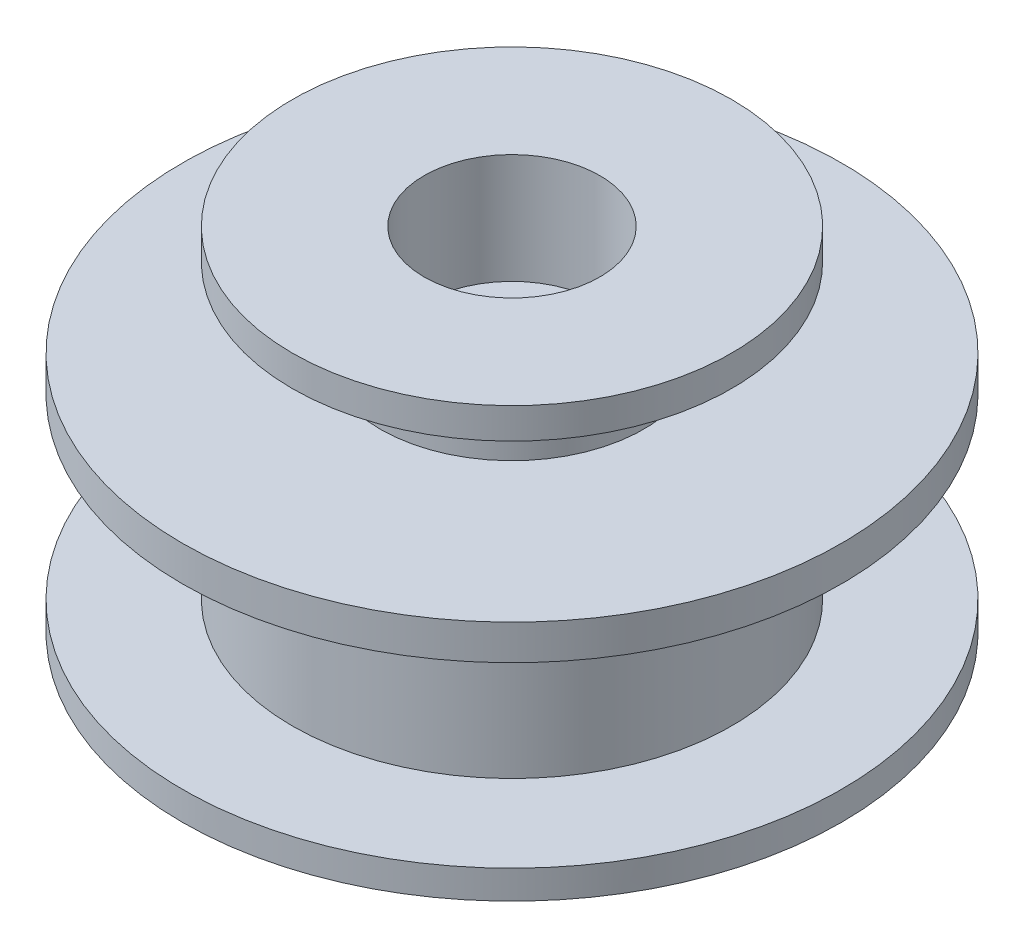
SolidWorks part; units mm, degrees
ref_plane "Front Plane" through (0, 0, 0) normal (0, 0, 1) x (1, 0, 0)
ref_plane "Top Plane" through (0, 0, 0) normal (0, 1, 0) x (1, 0, 0)
ref_plane "Right Plane" through (0, 0, 0) normal (1, 0, 0) x (0, 0, -1)
other "Configuration Table"
sketch "Sketch1" plane through (0, 0, 0) normal (0, 1, 0) x (1, 0, 0)
  circle A0 centre (0, 0) radius 7.5
  dimension "D1" = 15
extrude "Boss-Extrude1" add sketch "Sketch1" along normal blind 4
sketch "Sketch3" plane through (0, 0, 0) normal (0, 0, 1) x (1, 0, 0)
  line L0 (7.5, 0) -> (7.5, 4) construction
  line L1 (7.5, 3.9) -> (4.5, 3.9)
  line L2 (7.5, 3.9) -> (7.5, 0.65)
  line L3 (7.5, 0.65) -> (4.5, 0.65)
  line L4 (4.5, 3.9) -> (4.5, 0.65)
  line L5 (7.5, 4) -> (-7.5, 4) construction
  line L6 (-7.5, 0) -> (7.5, 0) construction
  line L7 (0, 0) -> (0, 7.7691) construction
  dimension "D1" = 0.1
  dimension "D2" = 0.65
  dimension "D3" = 3
revolve "Cut-Revolve1" cut sketch "Sketch3" angle 360 about L7
sketch "Sketch4" plane through (0, 0, 0) normal (0, 1, 0) x (1, 0, 0)
  circle A0 centre (0, 0) radius 5
  dimension "D1" = 10
extrude "Boss-Extrude2" add sketch "Sketch4" along normal blind 8
sketch "Sketch5" plane through (0, 0, 0) normal (0, 0, 1) x (1, 0, 0)
  line L0 (5, 4) -> (5, 8) construction
  line L1 (5, 5.5) -> (3, 5.5)
  line L2 (5, 5.5) -> (5, 7.3)
  line L3 (5, 7.3) -> (3, 7.3)
  line L4 (3, 5.5) -> (3, 7.3)
  line L5 (5, 8) -> (-5, 8) construction
  line L6 (7.5, 4) -> (-7.5, 4) construction
  line L7 (0, 4) -> (0, 7.4809) construction
  dimension "D1" = 0.7
  dimension "D2" = 1.5
  dimension "D3" = 2
revolve "Cut-Revolve2" cut sketch "Sketch5" angle 360 about L7
sketch "Sketch6" plane through (0, 8, 0) normal (0, 1, 0) x (1, 0, 0)
  circle A0 centre (0, 0) radius 2
  dimension "D1" = 4
extrude "Cut-Extrude1" cut sketch "Sketch6" against normal through all
sketch "Sketch7" plane through (0, 4, 0) normal (0, 1, 0) x (1, 0, 0)
  circle A0 centre (0, 0) radius 8.5721
  circle A1 centre (0, 0) radius 5
extrude "Cut-Extrude3" cut sketch "Sketch7" against normal blind 2
sketch "Sketch8" plane through (0, 5.5, 0) normal (0, 1, 0) x (1, 0, 0)
  circle A0 centre (0, 0) radius 7.5
  circle A1 centre (0, 0) radius 7.5 construction
  circle A2 centre (0, 0) radius 5
extrude "Boss-Extrude3" add sketch "Sketch8" against normal blind 0.8 contours A0
